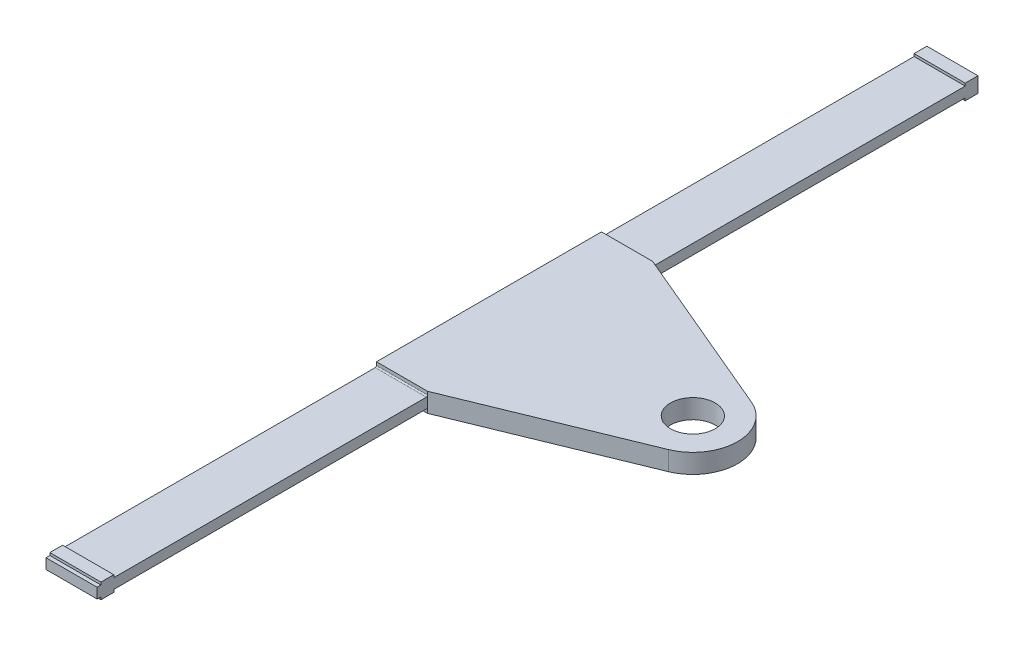
from build123d import *

# Parameters (mm, degrees)
SKETCH_1_W               = 40
SKETCH_1_H               = 8
EXTRUDE_1_DEPTH          = 330.5
EXTRUDE_START            = -4
EXTRUDE_9_DEPTH          = 7.5
CUT_EXTRUDE_1_DEPTH      = 375.443041078
CUT_EXTRUDE_1_DEPTH_BACK = 375.443041078
SKETCH_14_R              = 17.5
EXTRUDE_10_DEPTH         = 40
SKETCH_16_W              = 176
SKETCH_16_H              = 3.5
EXTRUDE_11_DEPTH         = 40
SKETCH_17_W              = 176
SKETCH_17_H              = 3.5
EXTRUDE_12_DEPTH         = 40
FILLET_1_R               = 1
CUT_EXTRUDE_2_DEPTH      = 398.850950952
CUT_EXTRUDE_2_DEPTH_BACK = 398.850950952
EXTRUDE_13_DEPTH         = 40


with BuildPart() as part:
    # 草图1 → 凸台-拉伸1 (new, symmetric)
    with BuildSketch(Plane.XY):
        Rectangle(SKETCH_1_W, SKETCH_1_H)
    extrude(amount=EXTRUDE_1_DEPTH, both=True)

    # 草图13 → 凸台-拉伸9 (add, symmetric)
    with BuildSketch(Plane.XZ.offset(4).offset(EXTRUDE_START)):
        with BuildLine():
            Line((153.622249649, 33.30434644), (20, 88))
            Line((20, 88), (20, -88))
            Line((20, -88), (153.998078719, -31.322105093))
            ThreePointArc((153.998078719, -31.322105093), (175.362862221, 1.116458369), (153.622249649, 33.30434644))
        make_face()
    extrude(amount=EXTRUDE_9_DEPTH, both=True)

    # 草图14 → 切除-拉伸1 (cut, two sides: drawn at the far end of the back side and taken through both)
    with BuildSketch(Plane.XZ.offset(7.5).offset(-CUT_EXTRUDE_1_DEPTH_BACK)):
        with Locations(Location((140.363454038, 0.912922591, 0), (0, 0, 270))):
            Circle(SKETCH_14_R)
    extrude(amount=CUT_EXTRUDE_1_DEPTH + CUT_EXTRUDE_1_DEPTH_BACK, mode=Mode.SUBTRACT)

    # 草图15 → 凸台-拉伸10 (add)
    with BuildSketch(Plane.ZY.offset(20)):
        Polygon((330.5, 4), (333.5, 4), (333.5, 6), (343.5, 6), (343.5, 4), (346.5, 4), (346.5, 0.516928803), (346.5, -4), (343.5, -4), (343.5, -6), (333.5, -6), (333.5, -4), (330.5, -4), align=None)
    extrude_10 = extrude(amount=-EXTRUDE_10_DEPTH)

    # 草图16 → 凸台-拉伸11 (add)
    with BuildSketch(Plane.ZY.offset(-20)):
        with Locations((0, 5.75)):
            Rectangle(SKETCH_16_W, SKETCH_16_H)
    extrude(amount=EXTRUDE_11_DEPTH)

    # 草图17 → 凸台-拉伸12 (add)
    with BuildSketch(Plane.ZY.offset(-20)):
        with Locations((0, -5.75)):
            Rectangle(SKETCH_17_W, SKETCH_17_H)
    extrude(amount=EXTRUDE_12_DEPTH)

    # 镜向1: 凸台-拉伸10 across plane
    add(extrude_10.mirror(Plane.XY))

    # 圆角1
    fillet_1_edges = [part.edges().sort_by_distance(p)[0] for p in [
        (0, 4, 88),
        (0, 4, -88),
        (0, -4, -88),
        (0, -4, 88),
    ]]
    fillet(fillet_1_edges, radius=FILLET_1_R)

    # 草图18 → 切除-拉伸2 (cut, two sides: drawn at the far end of the back side and taken through both)
    with BuildSketch(Plane.ZY.offset(20).offset(-CUT_EXTRUDE_2_DEPTH_BACK)):
        Polygon((-339.5, 4), (-339.5, 6), (-343.5, 6), (-343.5, 4), (-346.5, 4), (-346.5, -4), (-343.5, -4), (-343.5, -6), (-339.5, -6), (-339.5, -4), (-342.5, -4), (-342.5, 4), align=None)
    extrude(amount=CUT_EXTRUDE_2_DEPTH + CUT_EXTRUDE_2_DEPTH_BACK, mode=Mode.SUBTRACT)

    # 草图19 → 凸台-拉伸13 (add)
    with BuildSketch(Plane.ZY.offset(20)):
        Polygon((-332.5, 4), (-332.5, 6), (-342.5, 6), (-342.5, -6), (-332.5, -6), (-332.5, -4), align=None)
    extrude(amount=-EXTRUDE_13_DEPTH)


solid = part.part
